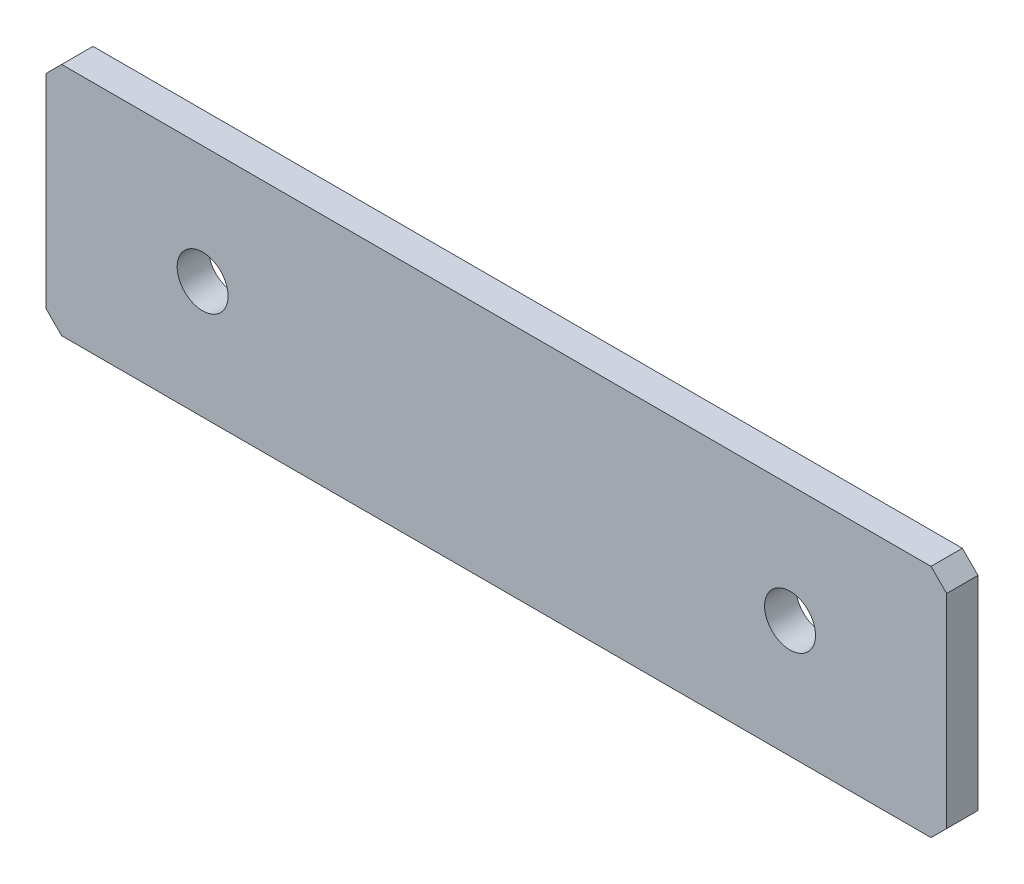
SolidWorks part; units mm, degrees
material "1023 碳钢板 (SS)"
ref_plane "Front Plane" through (0, 0, 0) normal (0, 0, 1) x (1, 0, 0)
ref_plane "Top Plane" through (0, 0, 0) normal (0, 1, 0) x (1, 0, 0)
ref_plane "Right Plane" through (0, 0, 0) normal (1, 0, 0) x (0, 0, -1)
sketch "Sketch1" plane through (0, 0, 0) normal (0, 0, 1) x (1, 0, 0)
  line L1 (57.5, 15) -> (-57.5, 15)
  line L2 (57.5, 15) -> (57.5, -15)
  line L3 (57.5, -15) -> (-57.5, -15)
  line L4 (-57.5, 15) -> (-57.5, -15)
  line L5 (57.5, 15) -> (-57.5, -15) construction
  line L6 (57.5, -15) -> (-57.5, 15) construction
  circle A0 centre (-37.5, 0) radius 3.25
  circle A1 centre (37.5, 0) radius 3.25
  point P0 (0, 0)
  dimension "D4" = 75
  dimension "D5" = 6.5
  dimension "D1" = 115
  dimension "D2" = 30
  dimension "D3" = 20
extrude "Boss-Extrude1" add sketch "Sketch1" along normal blind 4
chamfer "Chamfer1" distance 2 angle 45 4 edges at (-57.5, -15, 2) (-57.5, 15, 2) (57.5, -15, 2) (57.5, 15, 2)
